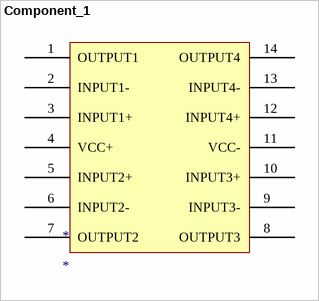
[diagram p0: symbol Component_1]
# Altium schematic symbol library MISC89340-16.SchLib: 1 symbol
Pins are listed as number, name and electrical type; pins without a type are passive.


## Component_1
designator *
footprint TL084
pins: 1 OUTPUT1, 2 INPUT1-, 3 INPUT1+, 4 VCC+, 5 INPUT2+, 6 INPUT2-, 7 OUTPUT2, 8 OUTPUT3, 9 INPUT3-, 10 INPUT3+, 11 VCC-, 12 INPUT4+, 13 INPUT4-, 14 OUTPUT4